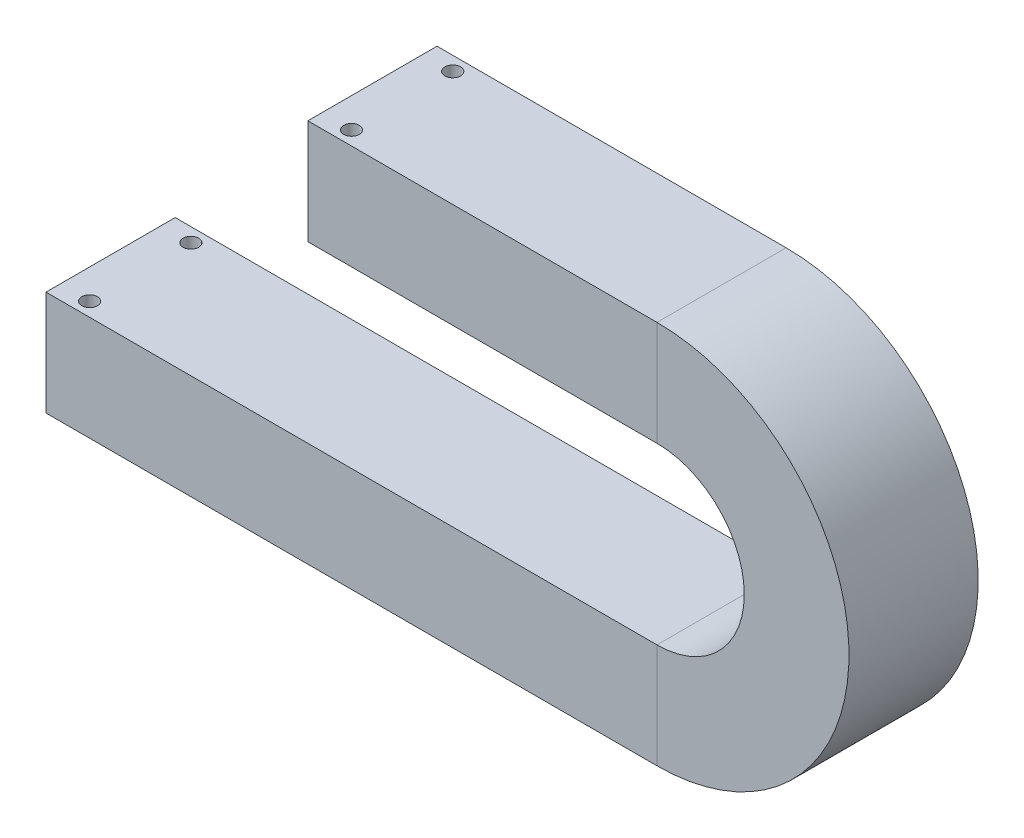
SolidWorks part; units mm, degrees
material "6061-T6"
ref_plane "Front Plane" through (0, 0, 0) normal (0, 0, 1) x (1, 0, 0)
ref_plane "Top Plane" through (0, 0, 0) normal (0, 1, 0) x (1, 0, 0)
ref_plane "Right Plane" through (0, 0, 0) normal (1, 0, 0) x (0, 0, -1)
sketch "Sketch1" plane through (0, 0, 0) normal (1, 0, 0) x (0, 0, -1)
  line L1 (-10, -10) -> (10, -10)
  line L2 (-10, -10) -> (-10, 10)
  line L3 (-10, 10) -> (10, 10)
  line L4 (10, -10) -> (10, 10)
  line L5 (-10, -10) -> (10, 10) construction
  line L6 (-10, 10) -> (10, -10) construction
  line L7 (-18.5, -15) -> (18.5, -15)
  line L8 (-18.5, -15) -> (-18.5, 15)
  line L9 (-18.5, 15) -> (18.5, 15)
  line L10 (18.5, -15) -> (18.5, 15)
  line L11 (-18.5, -15) -> (18.5, 15) construction
  line L12 (-18.5, 15) -> (18.5, -15) construction
  point P0 (0, 0)
  point P6 (0, 0)
  dimension "D1" = 20
  dimension "D2" = 20
  dimension "D3" = 30
  dimension "D4" = 37
sketch "Sketch2" plane through (0, 0, 0) normal (0, 0, 1) x (1, 0, 0)
  line L0 (0, 0) -> (175, 0)
  line L1 (175, 80) -> (75, 80)
  arc A0 (175, 0) -> (175, 80) centre (175, 40) ccw
  dimension "D1" = 80
  dimension "D2" = 175
  dimension "D3" = 100
sweep "Sweep1" add profiles "Sketch1" path "Sketch2"
hole_wizard "M4 Clearance Hole1" positions "Sketch3" profile "Sketch4" hole size "M4" standard "GB" end condition through all
sketch "Sketch3" plane through (0, 15, 0) normal (0, 1, 0) x (1, 0, 0)
  line L0 (0, 0) -> (230, 0) construction
  line L1 (230, -18.5) -> (230, 18.5) construction
  line L3 (0, 18.5) -> (0, -18.5) construction
  point P0 (8.5, 14.5)
  point P2 (8.5, -14.5)
  dimension "D1" = 29
  dimension "D2" = 8.5
sketch "Sketch4" plane through (8.5, 15, -14.5) normal (1, 0, 0) x (0, 0, 1)
  line L0 (0, 0) -> (0, 30)
  line L1 (0, 30) -> (2.25, 30)
  line L2 (2.25, 30) -> (2.25, 0)
  line L5 (2.25, 0) -> (0, 0)
  line L11 (0, -6.35) -> (0, 107.95) construction
  dimension "通孔孔直径" = 4.5
  dimension "通孔孔深度" = 30
hole_wizard "M4 Clearance Hole2" positions "Sketch5" profile "Sketch6" hole size "M4" standard "GB"
sketch "Sketch5" plane through (0, 95, 0) normal (0, 1, 0) x (1, 0, 0)
  line L0 (75, 0) -> (230, 0) construction
  line L1 (75, -18.5) -> (75, 18.5) construction
  line L2 (230, -18.5) -> (230, 18.5) construction
  point P8 (83.5, 14.5)
  point P10 (83.5, -14.5)
  dimension "D1" = 29
  dimension "D2" = 8.5
sketch "Sketch6" plane through (83.5, 95, 14.5) normal (1, 0, 0) x (0, 0, 1)
  line L0 (0, 0) -> (0, 51.3519)
  line L1 (0, 51.3519) -> (2.25, 50)
  line L2 (2.25, 50) -> (2.25, 0)
  line L5 (2.25, 0) -> (0, 0)
  line L10 (0, 51.3519) -> (-2.25, 50) construction
  line L11 (0, -6.35) -> (0, 107.95) construction
  dimension "孔直径" = 4.5
  dimension "孔深度" = 50
  dimension "导头角度" = 118
